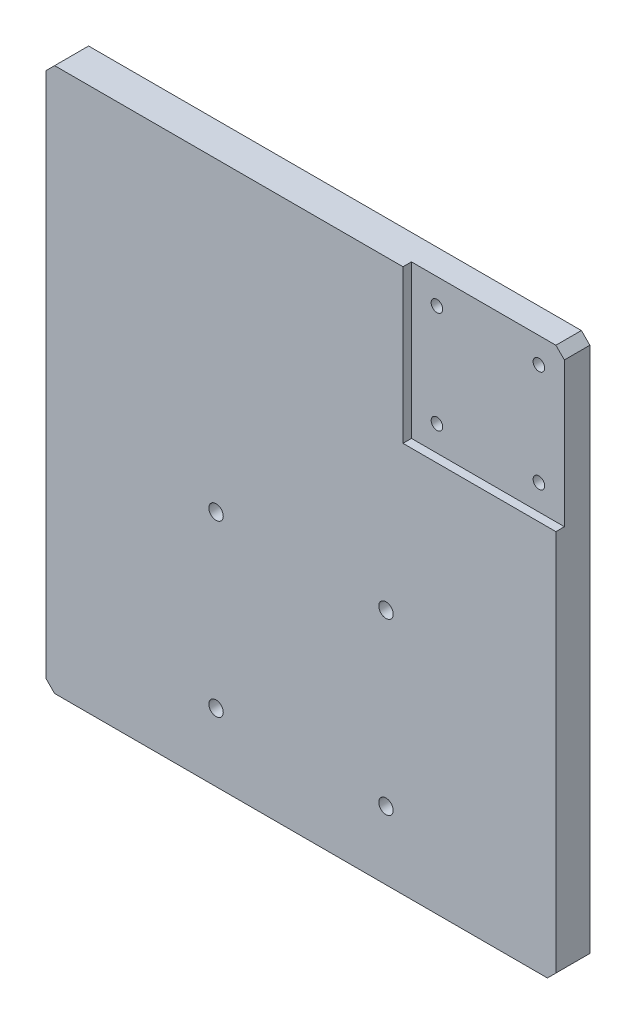
from build123d import *

# Parameters (mm, degrees)
SKETCH_1_W              = 300
SKETCH_1_H              = 320
EXTRUDE_1_DEPTH         = 10
HOLE_WIZARD_M10_1_D     = 8.5
HOLE_WIZARD_M10_1_DEPTH = 15
HOLE_WIZARD_M10_1_TIP   = 2.553657631
SKETCH_7_W              = 90
SKETCH_7_H              = 90
CUT_EXTRUDE_1_DEPTH     = 5
HOLE_WIZARD_M8_1_D      = 6.8
HOLE_WIZARD_M8_1_DEPTH  = 10
HOLE_WIZARD_M8_1_TIP    = 2.042926105
CHAMFER_1_SIZE          = 5


with BuildPart() as part:
    # 草图1 → 凸台-拉伸1 (new, symmetric)
    with BuildSketch(Plane.XY):
        Rectangle(SKETCH_1_W, SKETCH_1_H)
    extrude(amount=EXTRUDE_1_DEPTH, both=True)

    # M10 螺纹孔1
    with Locations(Plane.XY.offset(10)):
        with Locations((50, -20), (-50, -120), (-50, -20), (50, -120)):
            Hole(HOLE_WIZARD_M10_1_D / 2, depth=HOLE_WIZARD_M10_1_DEPTH)
            with Locations((0, 0, -(HOLE_WIZARD_M10_1_DEPTH + HOLE_WIZARD_M10_1_TIP / 2))):  # 118° drill point
                Cone(0, HOLE_WIZARD_M10_1_D / 2, HOLE_WIZARD_M10_1_TIP, mode=Mode.SUBTRACT)

    # 草图7 → 切除-拉伸1 (cut)
    with BuildSketch(Plane.XY.offset(10)):
        with Locations((105, 115)):
            Rectangle(SKETCH_7_W, SKETCH_7_H)
    extrude(amount=-CUT_EXTRUDE_1_DEPTH, mode=Mode.SUBTRACT)

    # M8 螺纹孔1
    with Locations(Plane.XY.offset(5)):
        with Locations((135, 145), (75, 85), (75, 145), (135, 85)):
            Hole(HOLE_WIZARD_M8_1_D / 2, depth=HOLE_WIZARD_M8_1_DEPTH)
            with Locations((0, 0, -(HOLE_WIZARD_M8_1_DEPTH + HOLE_WIZARD_M8_1_TIP / 2))):  # 118° drill point
                Cone(0, HOLE_WIZARD_M8_1_D / 2, HOLE_WIZARD_M8_1_TIP, mode=Mode.SUBTRACT)

    # 倒角1
    chamfer_1_edges = [part.edges().sort_by_distance(p)[0] for p in [
        (150, 160, -2.5),
        (150, -160, 0),
        (-150, -160, 0),
        (-150, 160, 0),
    ]]
    chamfer(chamfer_1_edges, length=CHAMFER_1_SIZE)


solid = part.part
